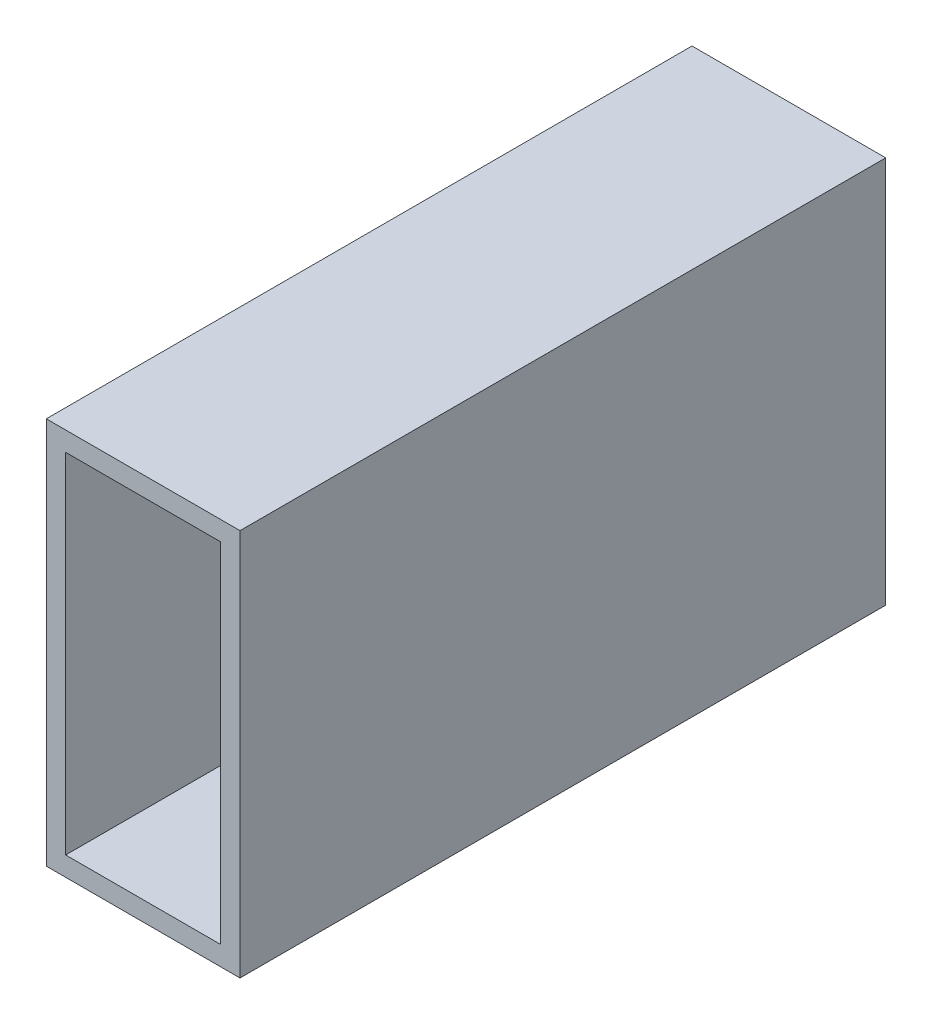
from build123d import *

# Parameters (mm, degrees)
SKETCH_1_W      = 30
SKETCH_1_H      = 60
SKETCH_1_W_2    = 24
SKETCH_1_H_2    = 54
EXTRUDE_1_DEPTH = 100


with BuildPart() as part:
    # 草图1 → 拉伸-薄壁1 (new body)
    with BuildSketch(Plane.XY):
        Rectangle(SKETCH_1_W, SKETCH_1_H)
        Rectangle(SKETCH_1_W_2, SKETCH_1_H_2, mode=Mode.SUBTRACT)
    extrude(amount=EXTRUDE_1_DEPTH)


solid = part.part
